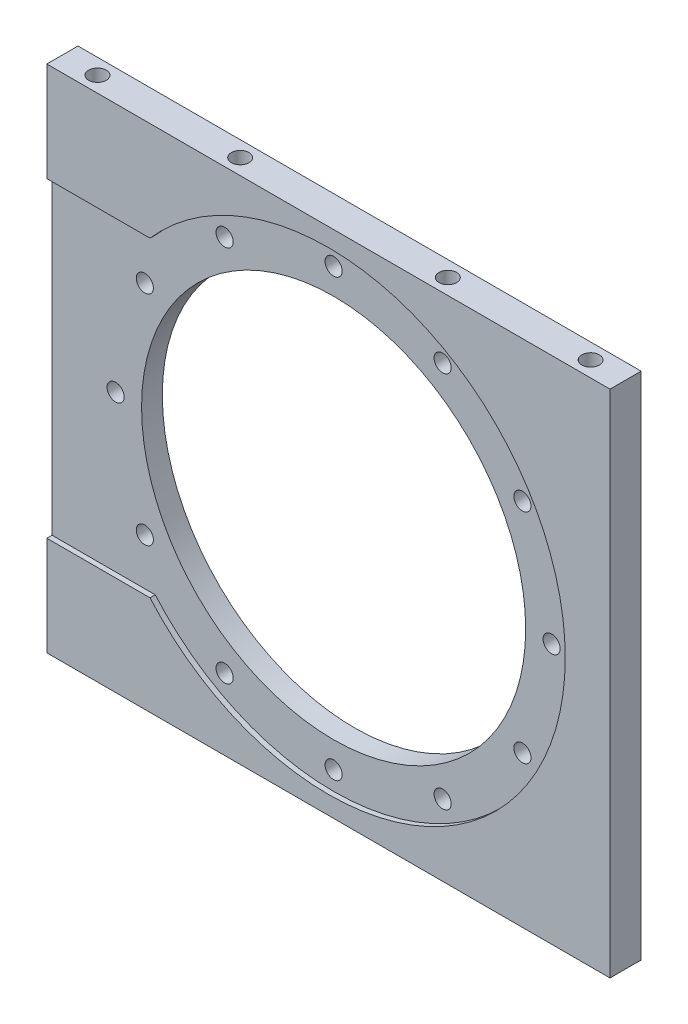
SolidWorks part; units mm, degrees
material "Q235A"
ref_plane "前视基准面" through (0, 0, 0) normal (0, 0, 1) x (1, 0, 0)
ref_plane "上视基准面" through (0, 0, 0) normal (0, 1, 0) x (1, 0, 0)
ref_plane "右视基准面" through (0, 0, 0) normal (1, 0, 0) x (0, 0, -1)
sketch "草图1" plane through (0, 0, 0) normal (0, 0, 1) x (1, 0, 0)
  line L1 (-108.5, -98.25) -> (108.5, -98.25)
  line L2 (-108.5, -98.25) -> (-108.5, 98.25)
  line L3 (-108.5, 98.25) -> (108.5, 98.25)
  line L4 (108.5, -98.25) -> (108.5, 98.25)
  line L5 (-108.5, -98.25) -> (108.5, 98.25) construction
  line L6 (-108.5, 98.25) -> (108.5, -98.25) construction
  circle A0 centre (0, 0) radius 74
  point P0 (0, 0)
  dimension "D3" = 148
  dimension "D1" = 217
  dimension "D2" = 196.5
extrude "凸台-拉伸1" add sketch "草图1" along normal blind 12
sketch "草图2" plane through (0, 0, 0) normal (0, 0, -1) x (-1, 0, 0)
  circle A0 centre (0, 0) radius 91.25
  dimension "D1" = 182.5
extrude "切除-拉伸1" cut sketch "草图2" against normal blind 2
sketch "草图3" plane through (0, 0, 12) normal (0, 0, 1) x (1, 0, 0)
  circle A1 centre (0, 0) radius 91.25
  circle A2 centre (0, 0) radius 91.25
  dimension "D1" = 0
extrude "切除-拉伸2" cut sketch "草图3" against normal blind 2
sketch "草图4" plane through (0, 0, 12) normal (0, 0, 1) x (1, 0, 0)
  line L0 (-108.5, 98.25) -> (-108.5, -98.25) construction
  line L1 (-68.75, 60) -> (-108.5, 60)
  line L2 (-68.75, 60) -> (-68.75, -60)
  line L3 (-68.75, -60) -> (-108.5, -60)
  line L4 (-108.5, 60) -> (-108.5, -60)
  circle A0 centre (0, 0) radius 91.25 construction
  circle A1 centre (0, 0) radius 91.25 construction
  point P8 (-71.3191, -56.5207)
  dimension "D1" = 120
extrude "切除-拉伸3" cut sketch "草图4" against normal up to surface (2 mm away) up to face at (74, 0, 10)
hole_wizard "M6 间隙孔1" positions "草图5" profile "草图6" hole size "M6" standard "ISO" end condition through all
sketch "草图5" plane through (0, 0, 2) normal (0, 0, -1) x (-1, 0, 0)
  line L0 (0, 0) -> (0, 84) construction
  point P0 (0, 84)
  point P6 (42, 72.7461)
  point P7 (72.7461, 42)
  point P8 (84, 0)
  point P9 (72.7461, -42)
  point P10 (42, -72.7461)
  point P11 (0, -84)
  point P12 (-42, -72.7461)
  point P13 (-72.7461, -42)
  point P14 (-84, 0)
  point P15 (-72.7461, 42)
  point P16 (-42, 72.7461)
  point P19 (0, 0)
  point P21 (0, 0)
  point P22 (-1.1906, 83.9916)
  dimension "D2" = 84
  dimension "D1" = 12
sketch "草图6" plane through (0, 84, 2) normal (1, 0, 0) x (0, 1, 0)
  line L0 (0, 0) -> (0, 10)
  line L1 (0, 10) -> (3.3, 10)
  line L2 (3.3, 10) -> (3.3, 0)
  line L5 (3.3, 0) -> (0, 0)
  line L11 (0, -6.35) -> (0, 107.95) construction
  dimension "通孔孔直径" = 6.6
  dimension "通孔孔深度" = 10
hole_wizard "M8 螺纹孔1" positions "草图7" profile "草图8" tap size "M8" standard "ISO"
sketch "草图7" plane through (0, -98.25, 0) normal (0, -1, 0) x (-1, 0, 0)
  line L0 (0, 0) -> (0, -12) construction
  line L1 (108.5, -12) -> (-108.5, -12) construction
  line L2 (-108.5, -6) -> (108.5, -6)
  line L3 (-108.5, -12) -> (-108.5, 0) construction
  line L4 (108.5, -12) -> (108.5, 0) construction
  point P0 (-95, -6)
  point P2 (-40, -6)
  point P12 (40, -6)
  point P14 (95, -6)
  dimension "D1" = 190
  dimension "D2" = 80
sketch "草图8" plane through (95, -98.25, 6) normal (1, 0, 0) x (0, 0, -1)
  line L0 (0, 0) -> (0, 21.7929)
  line L1 (0, 21.7929) -> (3.4, 19.75)
  line L2 (3.4, 19.75) -> (3.4, 0)
  line L5 (3.4, 0) -> (0, 0)
  line L10 (0, 21.7929) -> (-3.4, 19.75) construction
  line L11 (0, -6.35) -> (0, 107.95) construction
  dimension "螺纹孔钻头直径" = 6.8
  dimension "螺纹孔钻头深度" = 19.75
  dimension "导头角度" = 118
cosmetic thread "孔螺蚊线1" parameters "D1"=16, "D2"=8
cosmetic thread "孔螺蚊线2" parameters "D1"=16, "D2"=8
cosmetic thread "孔螺蚊线3" parameters "D1"=16, "D2"=8
cosmetic thread "孔螺蚊线4" parameters "D1"=16, "D2"=8
hole_wizard "M8 螺纹孔2" positions "草图9" profile "草图10" tap size "M8" standard "ISO"
sketch "草图9" plane through (0, 98.25, 0) normal (0, 1, 0) x (1, 0, 0)
  point P0 (-95, -6)
  point P3 (-40, -6)
  point P6 (40, -6)
  point P9 (95, -6)
sketch "草图10" plane through (-95, 98.25, 6) normal (1, 0, 0) x (0, 0, 1)
  line L0 (0, 0) -> (0, 21.7929)
  line L1 (0, 21.7929) -> (3.4, 19.75)
  line L2 (3.4, 19.75) -> (3.4, 0)
  line L5 (3.4, 0) -> (0, 0)
  line L10 (0, 21.7929) -> (-3.4, 19.75) construction
  line L11 (0, -6.35) -> (0, 107.95) construction
  dimension "螺纹孔钻头直径" = 6.8
  dimension "螺纹孔钻头深度" = 19.75
  dimension "导头角度" = 118
cosmetic thread "孔螺蚊线5" parameters "D1"=16, "D2"=8
cosmetic thread "孔螺蚊线6" parameters "D1"=16, "D2"=8
cosmetic thread "孔螺蚊线7" parameters "D1"=16, "D2"=8
cosmetic thread "孔螺蚊线8" parameters "D1"=16, "D2"=8
